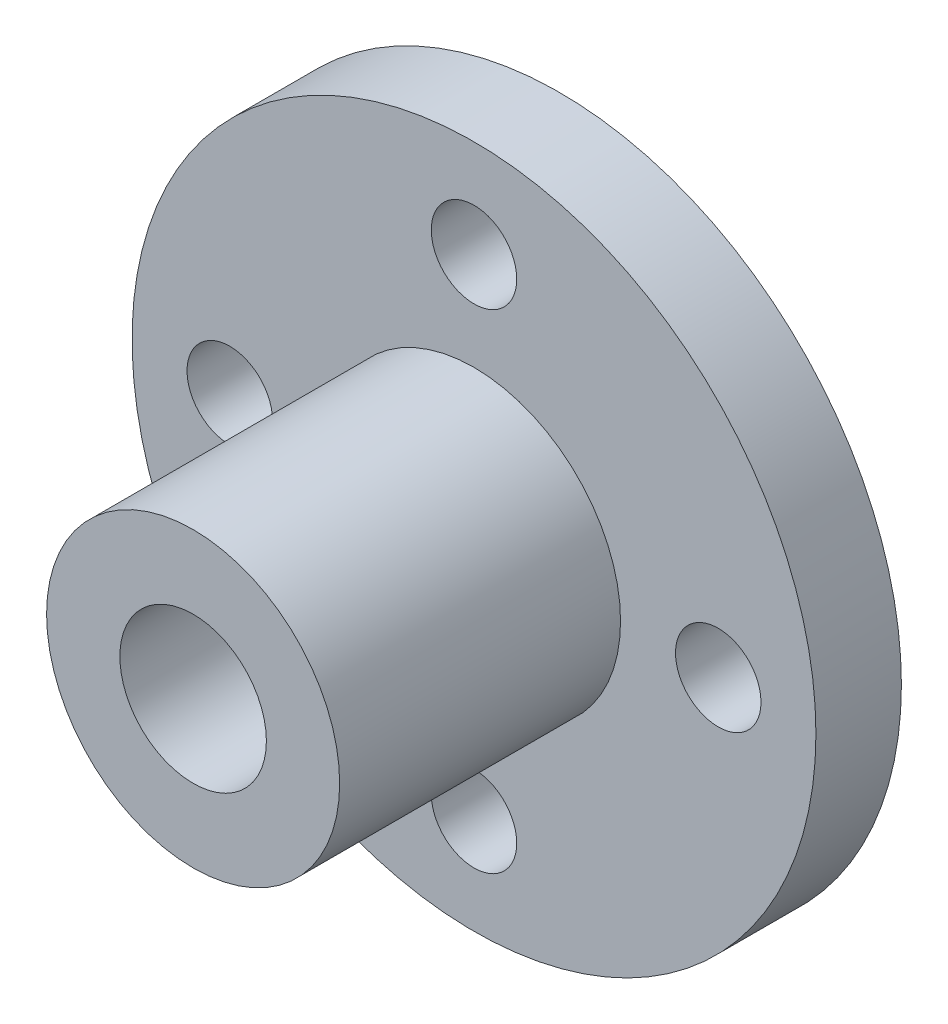
from build123d import *

# Parameters (mm, degrees)
SKETCH1_R           = 14
BOSS_EXTRUDE1_DEPTH = 3.5
SKETCH2_R           = 6
BOSS_EXTRUDE2_DEPTH = 11.5
SKETCH3_R           = 1.75
CUT_EXTRUDE1_DEPTH  = 11.5
CIRPATTERN1_COUNT   = 4
SKETCH4_R           = 3
CUT_EXTRUDE2_DEPTH  = 50


with BuildPart() as part:
    # Sketch1 → Boss-Extrude1 (new body)
    with BuildSketch(Plane.XY):
        Circle(SKETCH1_R)
    extrude(amount=BOSS_EXTRUDE1_DEPTH)

    # Sketch2 → Boss-Extrude2 (add)
    with BuildSketch(Plane.XY.offset(3.5)):
        Circle(SKETCH2_R)
    extrude(amount=BOSS_EXTRUDE2_DEPTH)

    # Sketch3 → Cut-Extrude1 (cut)
    with BuildSketch(Plane.XY.offset(3.5)):
        with Locations((0, 10)):
            Circle(SKETCH3_R)
    cut_extrude1 = extrude(amount=-CUT_EXTRUDE1_DEPTH, mode=Mode.SUBTRACT)

    # CirPattern1: Cut-Extrude1 ×4 about axis
    cirpattern1_axis = Axis((0, 0, 0), (0, 0, 1))
    for i in range(1, CIRPATTERN1_COUNT):
        add(cut_extrude1.rotate(cirpattern1_axis, i * 360 / CIRPATTERN1_COUNT), mode=Mode.SUBTRACT)

    # Sketch4 → Cut-Extrude2 (cut)
    with BuildSketch(Plane.XY.offset(15)):
        Circle(SKETCH4_R)
    extrude(amount=-CUT_EXTRUDE2_DEPTH, mode=Mode.SUBTRACT)


solid = part.part
